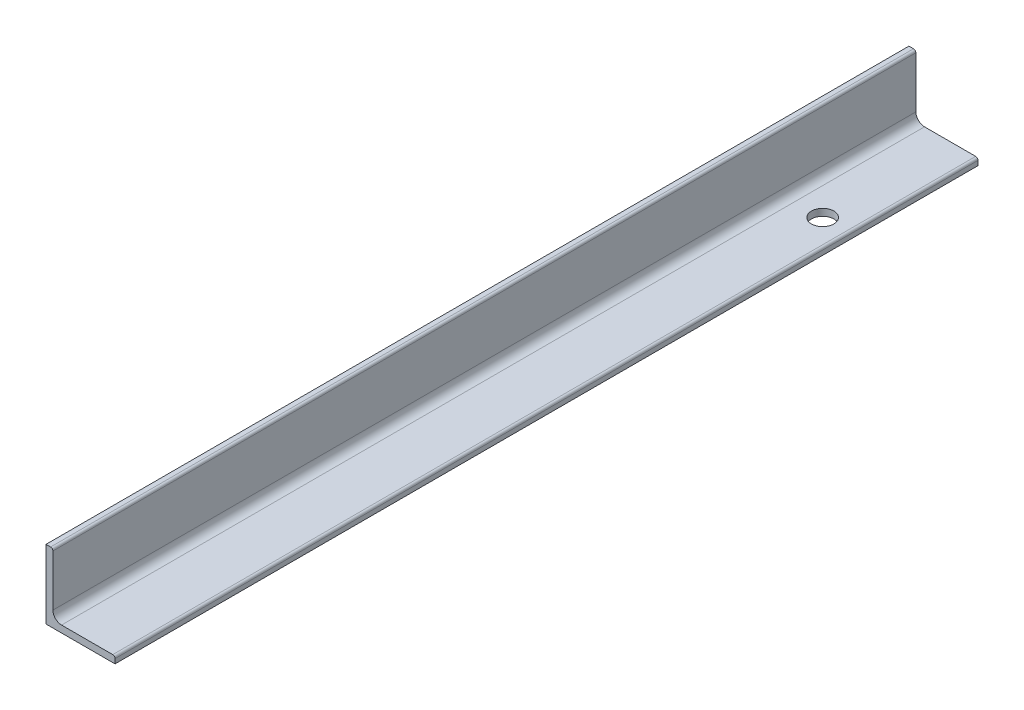
from build123d import *

# Parameters (mm, degrees)
BOSS_EXTRUDE1_DEPTH = 500
CUT_EXTRUDE1_REACH  = 504.888
SKETCH_1_R          = 6.5


with BuildPart() as part:
    # Sketch1 → Boss-Extrude1 (new body)
    with BuildSketch(Plane.XY):
        with BuildLine():
            Line((0, 0), (0, 40))
            Line((0, 40), (2.666666667, 40))
            ThreePointArc((2.666666667, 40), (3.609475708, 39.609475708), (4, 38.666666667))
            Line((4, 38.666666667), (4, 9))
            ThreePointArc((4, 9), (5.464466094, 5.464466094), (9, 4))
            Line((9, 4), (38.666666667, 4))
            ThreePointArc((38.666666667, 4), (39.609475708, 3.609475708), (40, 2.666666667))
            Line((40, 2.666666667), (40, 0))
            Line((40, 0), (0, 0))
        make_face()
    extrude(amount=BOSS_EXTRUDE1_DEPTH)

    # 草图1 → Cut-Extrude1 (cut, up to next)
    with BuildSketch(Plane(origin=(0, 4, 0), x_dir=(1, 0, 0), z_dir=(0, 1, 0)), mode=Mode.PRIVATE) as cut_extrude1_sk1:
        with Locations(Location((25, -75, 0), (0, 0, 180))):
            Circle(SKETCH_1_R)
    cut_extrude1_tool1 = extrude(cut_extrude1_sk1.sketch, amount=-CUT_EXTRUDE1_REACH, mode=Mode.PRIVATE) & part.part
    add(cut_extrude1_tool1.solids().sort_by_distance((25, 4, 75))[0], mode=Mode.SUBTRACT)


solid = part.part
